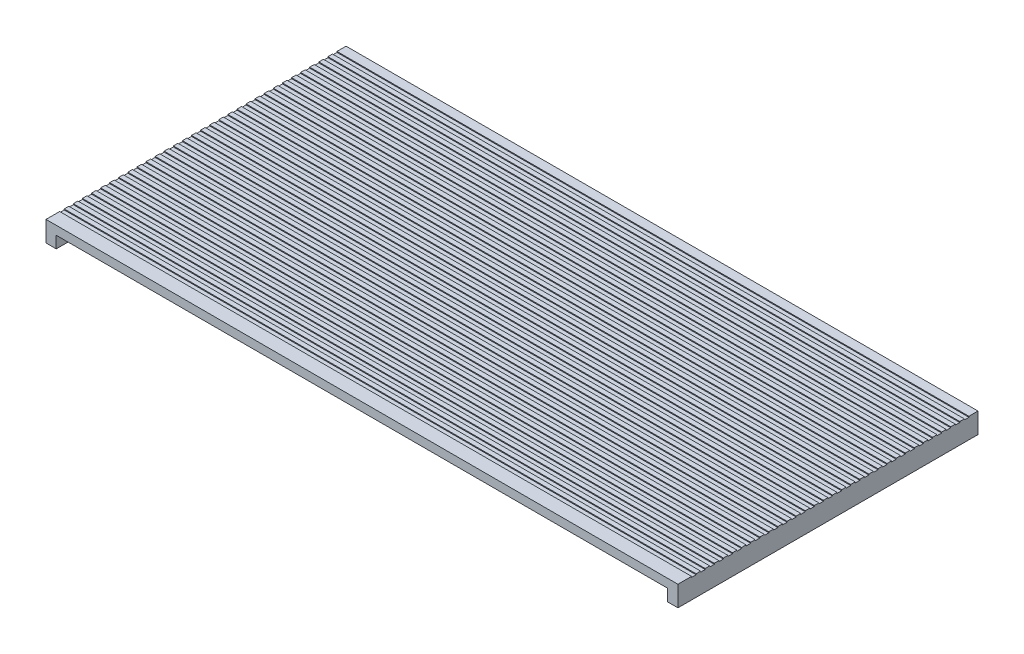
SolidWorks part; units mm, degrees
material "PE"
ref_plane "Front Plane" through (0, 0, 0) normal (0, 0, 1) x (1, 0, 0)
ref_plane "Top Plane" through (0, 0, 0) normal (0, 1, 0) x (1, 0, 0)
ref_plane "Right Plane" through (0, 0, 0) normal (1, 0, 0) x (0, 0, -1)
sketch "Sketch1" plane through (0, 0, 0) normal (0, 0, 1) x (1, 0, 0)
  line L0 (0, 22.5) -> (0, 3.5)
  line L1 (-695, 22.5) -> (695, 22.5)
  line L2 (-695, 22.5) -> (-695, -22.5)
  line L3 (-695, -22.5) -> (-672.5, -22.5)
  line L4 (695, 22.5) -> (695, -22.5)
  line L5 (-695, 22.5) -> (695, -22.5) construction
  line L6 (-695, -22.5) -> (695, 22.5) construction
  line L8 (-672.5, -22.5) -> (-672.5, 3.5)
  line L9 (-672.5, 3.5) -> (672.5, 3.5)
  line L10 (672.5, -22.5) -> (672.5, 3.5)
  line L11 (672.5, -22.5) -> (695, -22.5)
  point P0 (0, 0)
  dimension "D1" = 1390
  dimension "D2" = 45
  dimension "D3" = 1345
  dimension "D4" = 19
extrude "Boss-Extrude1" add sketch "Sketch1" along normal blind 660 contours L8 L9 L0 L1 L2 L3 | L10 L11 L4 L1 L0 L9
sketch "Sketch2" plane through (0, 22.5, 0) normal (0, 1, 0) x (1, 0, 0)
  line L0 (-695, -660) -> (-695, 0) construction
  line L1 (-695, -20) -> (695, -20)
  line L2 (-695, -20) -> (-695, -30)
  line L3 (-695, -30) -> (695, -30)
  line L4 (695, -20) -> (695, -30)
  line L5 (695, -660) -> (695, 0) construction
  line L6 (-695, 0) -> (695, 0) construction
  dimension "D1" = 20
  dimension "D2" = 10
extrude "Cut-Extrude1" cut sketch "Sketch2" against normal blind 2
pattern_linear "LPattern1" count 31 spacing 20 along (0, 0, 1) of "Cut-Extrude1"
